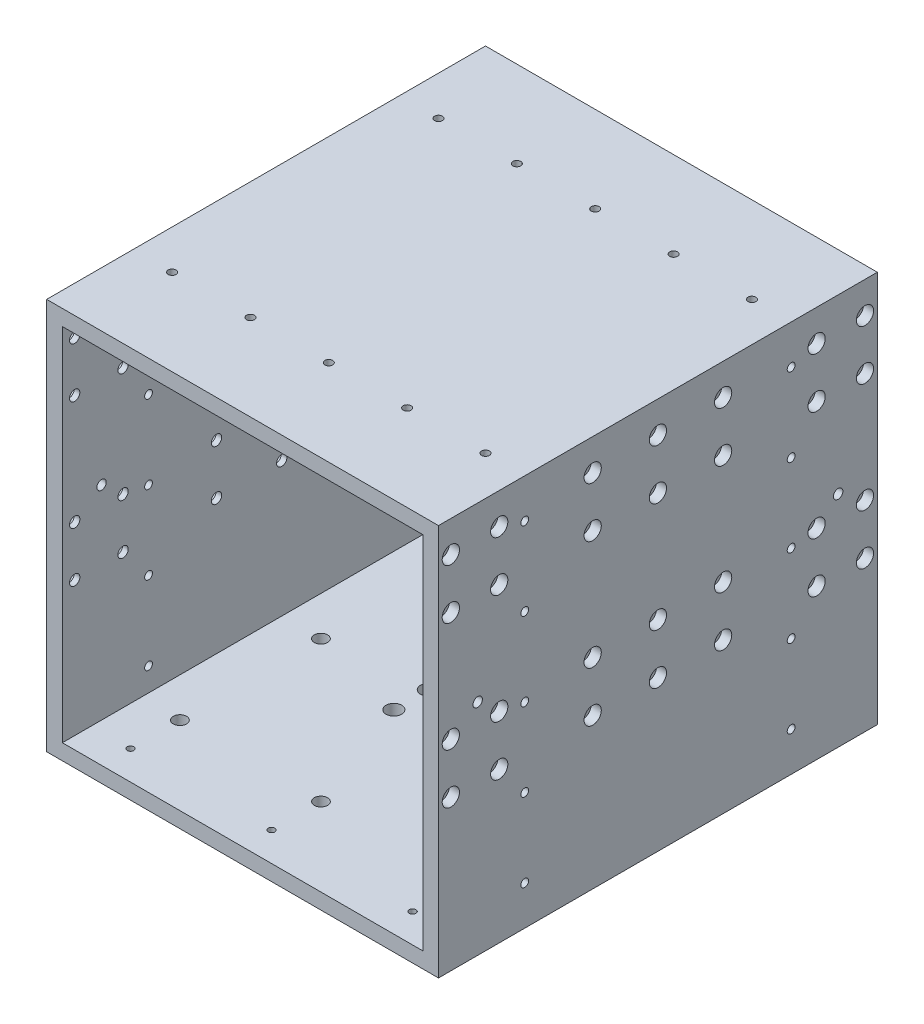
from build123d import *

# Parameters (mm, degrees)
SKETCH_1_W                   = 250
SKETCH_1_H                   = 250
SKETCH_1_W_2                 = 230
SKETCH_1_H_2                 = 230
EXTRUDE_1_DEPTH              = 140
HOLE_WIZARD_M10_1_D          = 8.5
HOLE_WIZARD_M10_1_DEPTH      = 10
HOLE_WIZARD_M6_1_D           = 6.6
HOLE_WIZARD_M6_1_DEPTH       = 10
HOLE_WIZARD_M6_1_CBORE_D     = 11
HOLE_WIZARD_M6_1_CBORE_DEPTH = 6.4
F_6_0MM_1_D                  = 6
HOLE_WIZARD_M8_1_D           = 10
HOLE_WIZARD_M8_1_DEPTH       = 10
CUT_EXTRUDE_2_REACH          = 314.61
SKETCH_13_R                  = 17.5
HOLE_WIZARD_M5_1_D           = 4.2
HOLE_WIZARD_M5_1_DEPTH       = 10
CHAMFER_1_SIZE               = 1
F_6_0MM_2_D                  = 6
F_6_0MM_2_DEPTH              = 8
F_6_0MM_2_TIP                = 1.802581857
HOLE_WIZARD_M6_1_2_D         = 5
HOLE_WIZARD_M6_2_D           = 5
HOLE_WIZARD_M6_2_DEPTH       = 10


with BuildPart() as part:
    # 草图1 → 凸台-拉伸1 (new, symmetric)
    with BuildSketch(Plane.XY):
        Rectangle(SKETCH_1_W, SKETCH_1_H)
        Rectangle(SKETCH_1_W_2, SKETCH_1_H_2, mode=Mode.SUBTRACT)
    extrude(amount=EXTRUDE_1_DEPTH, both=True)

    # M10 螺纹孔1
    with Locations(Plane.XZ.offset(125)):
        with Locations((-90, -90), (0, -90), (90, -90), (90, 0), (90, 90), (0, 90), (-90, 90), (-90, 0)):
            Hole(HOLE_WIZARD_M10_1_D / 2, depth=HOLE_WIZARD_M10_1_DEPTH)

    # Hole Wizard M6 _1
    with Locations(Plane.ZY.offset(125)):
        with Locations((-132.125, 3), (-132.125, -29), (-101.25, 3), (-101.25, -29), (-41.625, 3), (-41.625, -29), (0, 3), (0, -29), (41.625, -29), (41.625, 3), (101.25, -29), (101.25, 3), (132.125, -29), (132.125, 3), (-132.125, 73), (-132.125, 105), (-101.25, 105), (-101.25, 73), (-41.625, 105), (-41.625, 73), (0, 105), (0, 73), (41.625, 105), (41.625, 73), (101.25, 105), (101.25, 73), (132.125, 105), (132.125, 73)):
            hole_wizard_m6_1 = CounterBoreHole(HOLE_WIZARD_M6_1_D / 2, HOLE_WIZARD_M6_1_CBORE_D / 2, HOLE_WIZARD_M6_1_CBORE_DEPTH, depth=HOLE_WIZARD_M6_1_DEPTH)

    # 镜向1: Hole Wizard M6 _1 across plane
    add(hole_wizard_m6_1.mirror(Plane(origin=(0, 0, 0), x_dir=(0, 0, 1), z_dir=(1, 0, 0))), mode=Mode.SUBTRACT)

    # Ø6.0mm 暗销孔1 (through all)
    with Locations(Plane(origin=(125, 0, 0), x_dir=(0, 0, -1), z_dir=(1, 0, 0))):
        with Locations((-115, 15), (115, 15)):
            Hole(F_6_0MM_1_D / 2)

    # M8 间隙孔1
    with Locations(Plane(origin=(0, -125, 0), x_dir=(-1, 0, 0), z_dir=(0, -1, 0))):
        with Locations((-27.5, 6), (-27.5, -16), (0, 6), (0, -16), (27.5, 6), (27.5, -16)):
            Hole(HOLE_WIZARD_M8_1_D / 2, depth=HOLE_WIZARD_M8_1_DEPTH)

    # 草图13 → 切除-拉伸2 (cut, up to next)
    with BuildSketch(Plane.XZ.offset(125), mode=Mode.PRIVATE) as cut_extrude_2_sk1:
        with Locations(Location((85, -117.5, 0), (0, 0, 270))):
            Circle(SKETCH_13_R)
    cut_extrude_2_tool1 = extrude(cut_extrude_2_sk1.sketch, amount=-CUT_EXTRUDE_2_REACH, mode=Mode.PRIVATE) & part.part
    # 草图13 → 切除-拉伸2 (cut, up to next)
    with BuildSketch(Plane.XZ.offset(125), mode=Mode.PRIVATE) as cut_extrude_2_sk2:
        with Locations(Location((-85, -117.5, 0), (0, 0, 90))):
            Circle(SKETCH_13_R)
    cut_extrude_2_tool2 = extrude(cut_extrude_2_sk2.sketch, amount=-CUT_EXTRUDE_2_REACH, mode=Mode.PRIVATE) & part.part
    add(cut_extrude_2_tool1.solids().sort_by_distance((85, -125, -117.5))[0], mode=Mode.SUBTRACT)
    add(cut_extrude_2_tool2.solids().sort_by_distance((-85, -125, -117.5))[0], mode=Mode.SUBTRACT)

    # M5 螺纹孔1
    with Locations(Plane(origin=(0, -125, 0), x_dir=(-1, 0, 0), z_dir=(0, -1, 0))):
        with Locations((-90, -121.5), (0, -121.5), (90, -121.5)):
            Hole(HOLE_WIZARD_M5_1_D / 2, depth=HOLE_WIZARD_M5_1_DEPTH)

    # 倒角1
    chamfer_1_edges = [part.edges().sort_by_distance(p)[0] for p in [
        (85, -115, -100),
        (85, -125, -100),
        (-85, -115, -135),
        (-85, -125, -135),
    ]]
    chamfer(chamfer_1_edges, length=CHAMFER_1_SIZE)

    # Ø6.0mm 暗销孔2
    with Locations(Plane(origin=(0, -125, 0), x_dir=(-1, 0, 0), z_dir=(0, -1, 0))):
        with Locations((25, 88.75), (25, -88.75)):
            Hole(F_6_0MM_2_D / 2, depth=F_6_0MM_2_DEPTH)
            with Locations((0, 0, -(F_6_0MM_2_DEPTH + F_6_0MM_2_TIP / 2))):  # 118° drill point
                Cone(0, F_6_0MM_2_D / 2, F_6_0MM_2_TIP, mode=Mode.SUBTRACT)

    # Hole Wizard M6 _1 2 (through all)
    with Locations(Plane.ZY.offset(125)):
        with Locations((85, 0), (85, 50), (85, 100), (85, -100), (85, -50), (-85, -50), (-85, -100), (-85, 100), (-85, 50), (-85, 0)):
            Hole(HOLE_WIZARD_M6_1_2_D / 2)

    # M6 螺纹孔2
    with Locations(Plane(origin=(0, 125, 0), x_dir=(1, 0, 0), z_dir=(0, 1, 0))):
        with Locations((0, 85), (50, 85), (100, 85), (-100, 85), (-50, 85), (-50, -85), (-100, -85), (100, -85), (50, -85), (0, -85)):
            Hole(HOLE_WIZARD_M6_2_D / 2, depth=HOLE_WIZARD_M6_2_DEPTH)


solid = part.part
